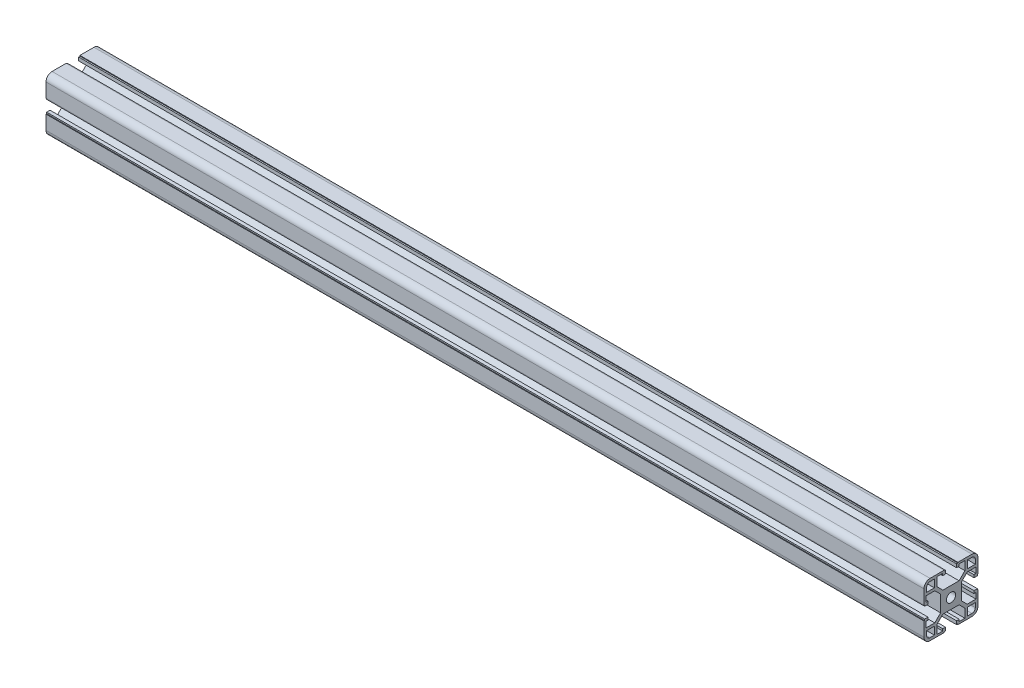
SolidWorks part; units mm, degrees
ref_plane "Front Plane" through (0, 0, 0) normal (0, 0, 1) x (1, 0, 0)
ref_plane "Top Plane" through (0, 0, 0) normal (0, 1, 0) x (1, 0, 0)
ref_plane "Right Plane" through (0, 0, 0) normal (1, 0, 0) x (0, 0, -1)
sketch "草图1" plane through (0, 0, 0) normal (0, 0, 1) x (1, 0, 0)
  line L0 (-984.975, 0) -> (-334.975, 0)
  dimension "D1" = 650
other "Aluminium profile 40 X 40B X R4.5(1)"
ref_plane "Plane1" through (-984.975, 0, 0) normal (1, 0, 0) x (0, 1, 0)
sketch "Sketch1" plane through (-984.975, 0, 0) normal (1, 0, 0) x (0, 1, 0)
  line L0 (-5.1, 20) -> (-5.1, 19.5)
  line L1 (-5.1, 19.5) -> (-4.1, 19.5)
  line L2 (-4.1, 19.5) -> (-4.1, 17)
  line L3 (-6.1, 18.5) -> (-10.3, 18.5)
  line L4 (-15.5, -20) -> (-5.1, -20)
  line L5 (-20, -15.5) -> (-20, -5.1)
  line L6 (15.5, 20) -> (5.1, 20)
  line L7 (20, 15.5) -> (20, 5.1)
  line L8 (0, 14.8756) -> (0, 0) construction
  line L9 (0, 0) -> (14.1675, 0) construction
  line L10 (-10.3, 18.5) -> (-10.3, 12)
  line L11 (-10.3, 12) -> (-6, 7.7)
  line L12 (-6, 7.7) -> (6, 7.7)
  line L13 (10.3, 12) -> (6, 7.7)
  line L14 (10.3, 18.5) -> (10.3, 12)
  line L15 (6.1, 18.5) -> (10.3, 18.5)
  line L16 (4.1, 19.5) -> (4.1, 17)
  line L17 (5.1, 19.5) -> (4.1, 19.5)
  line L18 (5.1, 20) -> (5.1, 19.5)
  line L19 (-5.1, 20) -> (-15.5, 20)
  line L20 (20, 5.1) -> (19.5, 5.1)
  line L21 (12.3, 18) -> (15.5, 18)
  line L22 (12.3, 18) -> (12.3, 12.3)
  line L23 (12.3, 12.3) -> (18, 12.3)
  line L24 (18, 15.5) -> (18, 12.3)
  line L25 (19.5, 5.1) -> (19.5, 4.1)
  line L26 (19.5, 4.1) -> (17, 4.1)
  line L27 (17, 6.1) -> (17, 4.1)
  line L28 (18.5, 6.1) -> (17, 6.1)
  line L29 (18.5, 6.1) -> (18.5, 10.3)
  line L30 (18.5, 10.3) -> (12, 10.3)
  line L31 (12, 10.3) -> (7.7, 6)
  line L32 (7.7, 6) -> (7.7, -6)
  line L33 (12, -10.3) -> (7.7, -6)
  line L34 (18.5, -10.3) -> (12, -10.3)
  line L35 (18.5, -6.1) -> (18.5, -10.3)
  line L36 (18.5, -6.1) -> (17, -6.1)
  line L37 (17, -4.1) -> (17, -6.1)
  line L38 (19.5, -4.1) -> (17, -4.1)
  line L39 (19.5, -5.1) -> (19.5, -4.1)
  line L40 (20, -5.1) -> (19.5, -5.1)
  line L41 (5.1, -20) -> (5.1, -19.5)
  line L42 (5.1, -19.5) -> (4.1, -19.5)
  line L43 (4.1, -19.5) -> (4.1, -17)
  line L44 (6.1, -17) -> (4.1, -17)
  line L45 (6.1, -18.5) -> (6.1, -17)
  line L46 (6.1, -18.5) -> (10.3, -18.5)
  line L47 (10.3, -18.5) -> (10.3, -12)
  line L48 (10.3, -12) -> (6, -7.7)
  line L49 (6, -7.7) -> (-6, -7.7)
  line L50 (-10.3, -12) -> (-6, -7.7)
  line L51 (-10.3, -18.5) -> (-10.3, -12)
  line L52 (-6.1, -18.5) -> (-10.3, -18.5)
  line L53 (-6.1, -18.5) -> (-6.1, -17)
  line L54 (-4.1, -17) -> (-6.1, -17)
  line L55 (-4.1, -19.5) -> (-4.1, -17)
  line L56 (-5.1, -19.5) -> (-4.1, -19.5)
  line L57 (-5.1, -20) -> (-5.1, -19.5)
  line L58 (-20, -5.1) -> (-19.5, -5.1)
  line L59 (5.1, -20) -> (15.5, -20)
  line L60 (-20, 5.1) -> (-20, 15.5)
  line L61 (-19.5, -5.1) -> (-19.5, -4.1)
  line L62 (-6.1, 18.5) -> (-6.1, 17)
  line L63 (-6.1, 17) -> (-4.1, 17)
  line L64 (6.1, 18.5) -> (6.1, 17)
  line L65 (4.1, 17) -> (6.1, 17)
  line L66 (-19.5, -4.1) -> (-17, -4.1)
  line L67 (-15.5, 18) -> (-12.3, 18)
  line L68 (-18, 15.5) -> (-18, 12.3)
  line L69 (-18, 12.3) -> (-12.3, 12.3)
  line L70 (-12.3, 18) -> (-12.3, 12.3)
  line L71 (-17, -6.1) -> (-17, -4.1)
  line L72 (-18.5, -6.1) -> (-17, -6.1)
  line L73 (-18.5, -6.1) -> (-18.5, -10.3)
  line L74 (-18.5, -10.3) -> (-12, -10.3)
  line L75 (-12, -10.3) -> (-7.7, -6)
  line L76 (-7.7, -6) -> (-7.7, 6)
  line L77 (-12, 10.3) -> (-7.7, 6)
  line L78 (-18.5, 10.3) -> (-12, 10.3)
  line L79 (-18.5, 6.1) -> (-18.5, 10.3)
  line L80 (-18.5, 6.1) -> (-17, 6.1)
  line L81 (-17, 4.1) -> (-17, 6.1)
  line L82 (-19.5, 4.1) -> (-17, 4.1)
  line L83 (-19.5, 5.1) -> (-19.5, 4.1)
  line L84 (-20, 5.1) -> (-19.5, 5.1)
  line L85 (20, -5.1) -> (20, -15.5)
  line L87 (-18, -12.3) -> (-12.3, -12.3)
  line L88 (-18, -12.3) -> (-18, -15.5)
  line L89 (-15.5, -18) -> (-12.3, -18)
  line L90 (-12.3, -12.3) -> (-12.3, -18)
  line L91 (12.3, -12.3) -> (18, -12.3)
  line L92 (12.3, -12.3) -> (12.3, -18)
  line L93 (12.3, -18) -> (15.5, -18)
  line L94 (18, -12.3) -> (18, -15.5)
  circle A0 centre (0, 0) radius 3.4
  arc A1 (-20, 15.5) -> (-15.5, 20) centre (-15.5, 15.5) cw
  arc A2 (20, 15.5) -> (15.5, 20) centre (15.5, 15.5) ccw
  arc A3 (-15.5, -20) -> (-20, -15.5) centre (-15.5, -15.5) cw
  arc A4 (15.5, -20) -> (20, -15.5) centre (15.5, -15.5) ccw
  arc A5 (-15.5, 18) -> (-18, 15.5) centre (-15.5, 15.5) ccw
  arc A6 (18, 15.5) -> (15.5, 18) centre (15.5, 15.5) ccw
  arc A7 (18, -15.5) -> (15.5, -18) centre (15.5, -15.5) cw
  arc A8 (-18, -15.5) -> (-15.5, -18) centre (-15.5, -15.5) ccw
  point P2 (0, 10)
  point P4 (0, 0)
  point P5 (-20, -20)
  point P6 (20, -20)
  point P7 (20, 20)
  point P8 (-20, 20)
  point P36 (-20, 20)
  point P39 (20, 20)
  point P121 (0, 0)
  dimension "D1" = 20.6
  dimension "D2" = 40
  dimension "D3" = 8.2
  dimension "D4" = 10.2
  dimension "D5" = 12.3
  dimension "D6" = 6.8
  dimension "D7" = 4.5
  dimension "D8" = 45
  dimension "D12" = 2
  dimension "D13" = 5.7
  dimension "D14" = 2
  dimension "D18" = 2.5
  dimension "D19" = 2.5
  dimension "D15" = 2.5
  dimension "D9" = 0.5
  dimension "D10" = 1.5
  dimension "D11" = 12
  dimension "D16" = 3
  dimension "D17" = 2
  dimension "D20" = 2
  dimension "D21" = 2
